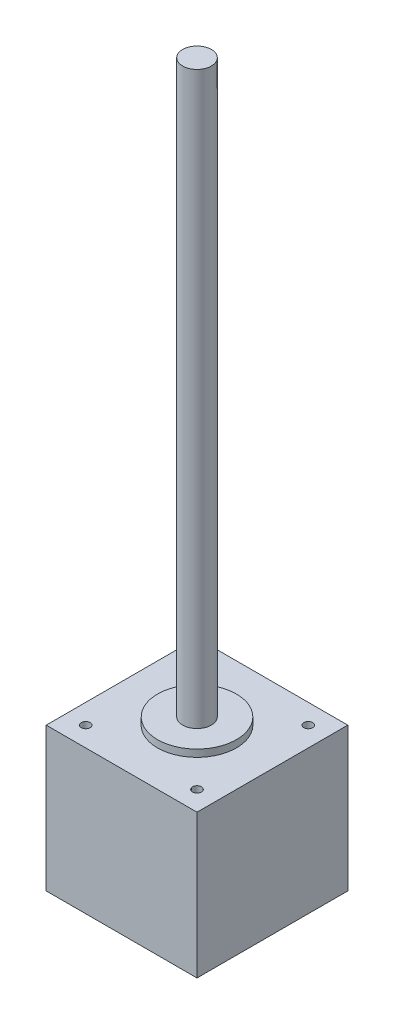
SolidWorks part; units mm, degrees
material "20#"
ref_plane "Front Plane" through (0, 0, 0) normal (0, 0, 1) x (1, 0, 0)
ref_plane "Top Plane" through (0, 0, 0) normal (0, 1, 0) x (1, 0, 0)
ref_plane "Right Plane" through (0, 0, 0) normal (1, 0, 0) x (0, 0, -1)
sketch "Sketch1" plane through (0, 0, 0) normal (0, 1, 0) x (1, 0, 0)
  line L1 (-21, 21) -> (21, 21)
  line L2 (-21, 21) -> (-21, -21)
  line L3 (-21, -21) -> (21, -21)
  line L4 (21, 21) -> (21, -21)
  line L5 (-21, 21) -> (21, -21) construction
  line L6 (-21, -21) -> (21, 21) construction
  point P0 (0, 0)
  dimension "D1" = 42
extrude "Boss-Extrude1" add sketch "Sketch1" along normal blind 40
sketch "Sketch2" plane through (0, 40, 0) normal (0, 1, 0) x (1, 0, 0)
  circle A0 centre (0, 0) radius 11
  dimension "D1" = 22
extrude "Boss-Extrude2" add sketch "Sketch2" along normal blind 2
sketch "Sketch3" plane through (0, 42, 0) normal (0, 1, 0) x (1, 0, 0)
  circle A0 centre (0, 0) radius 4
  dimension "D1" = 8
extrude "Boss-Extrude3" add sketch "Sketch3" along normal blind 159
cosmetic thread "Cosmetic Thread1" parameters "D2"=4.917
sketch "Sketch4" plane through (0, 40, 0) normal (0, 1, 0) x (1, 0, 0)
  line L1 (-15.5, 15.5) -> (15.5, 15.5) construction
  line L2 (-15.5, 15.5) -> (-15.5, -15.5) construction
  line L3 (-15.5, -15.5) -> (15.5, -15.5) construction
  line L4 (15.5, 15.5) -> (15.5, -15.5) construction
  line L5 (-15.5, 15.5) -> (15.5, -15.5) construction
  line L6 (-15.5, -15.5) -> (15.5, 15.5) construction
  circle A0 centre (-15.5, 15.5) radius 0.75
  circle A1 centre (15.5, 15.5) radius 0.75
  circle A2 centre (15.5, -15.5) radius 0.75
  circle A3 centre (-15.5, -15.5) radius 0.75
  point P0 (0, 0)
  dimension "D3" = 1.5
  dimension "D1" = 31
  dimension "D2" = 31
extrude "Cut-Extrude1" cut sketch "Sketch4" against normal blind 5
hole_wizard "M3 Tapped Hole1" positions "Sketch5" profile "Sketch6" tap size "M3" standard "GB"
sketch "Sketch5" plane through (0, 40, 0) normal (0, 1, 0) x (1, 0, 0)
  point P0 (-15.5, 15.5)
  point P9 (15.5, -15.5)
  point P12 (-15.5, -15.5)
  point P17 (15.5, 15.5)
sketch "Sketch6" plane through (-15.5, 40, -15.5) normal (1, 0, 0) x (0, 0, 1)
  line L0 (0, 0) -> (0, 8.2511)
  line L1 (0, 8.2511) -> (1.25, 7.5)
  line L2 (1.25, 7.5) -> (1.25, 0)
  line L5 (1.25, 0) -> (0, 0)
  line L10 (0, 8.2511) -> (-1.25, 7.5) construction
  line L11 (0, -6.35) -> (0, 107.95) construction
  dimension "螺纹孔钻头直径" = 2.5
  dimension "螺纹孔钻头深度" = 7.5
  dimension "导头角度" = 118
cosmetic thread "HoleThreadLine1" parameters "D1"=6, "D2"=3
cosmetic thread "HoleThreadLine2" parameters "D1"=6, "D2"=3
cosmetic thread "HoleThreadLine3" parameters "D1"=6, "D2"=3
cosmetic thread "HoleThreadLine4" parameters "D1"=6, "D2"=3
